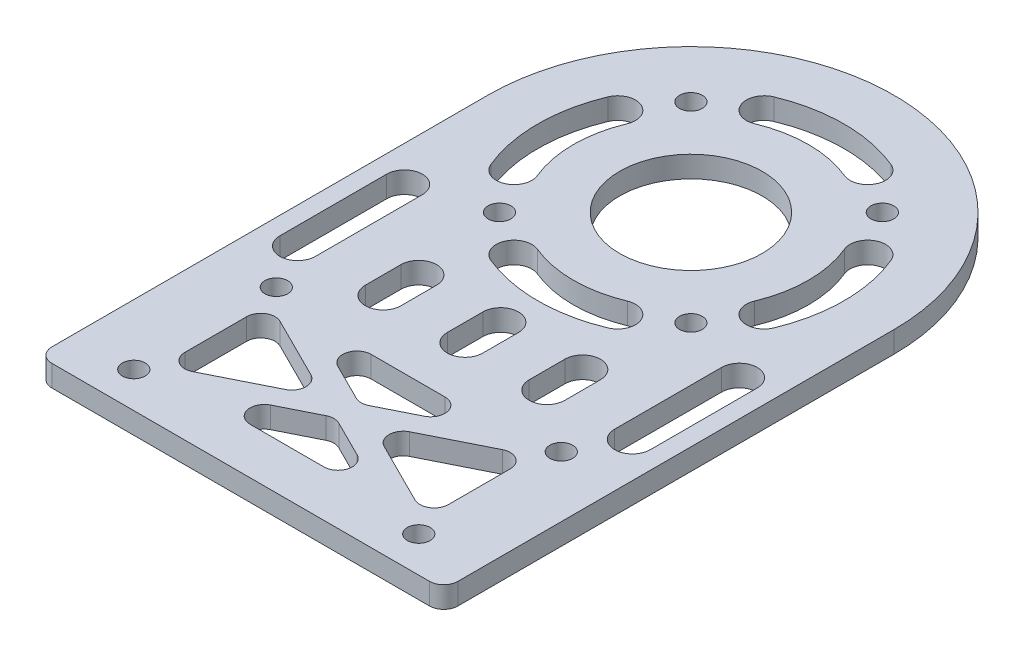
SolidWorks part; units mm, degrees
material "哈碳纤"
ref_plane "前视基准面" through (0, 0, 0) normal (0, 0, 1) x (1, 0, 0)
ref_plane "上视基准面" through (0, 0, 0) normal (0, 1, 0) x (1, 0, 0)
ref_plane "右视基准面" through (0, 0, 0) normal (1, 0, 0) x (0, 0, -1)
other "Configuration Table"
sketch "草图1" plane through (0, 0, 0) normal (0, 1, 0) x (1, 0, 0)
  line L0 (-20, -38.2) -> (20, -58.2) construction
  line L2 (-28.5, 0) -> (-28.5, -63.2)
  line L3 (-28.5, -63.2) -> (28.5, -63.2)
  line L4 (28.5, 0) -> (28.5, -63.2)
  line L5 (-20, -58.2) -> (20, -58.2) construction
  line L6 (-20, -58.2) -> (-20, -38.2) construction
  line L7 (-20, -38.2) -> (20, -38.2) construction
  line L8 (20, -58.2) -> (20, -38.2) construction
  line L9 (-19, 0) -> (0, 0) construction
  line L10 (0, 0) -> (-13.435, 13.435) construction
  arc A0 (28.5, 0) -> (-28.5, 0) centre (0, 0) ccw
  circle A1 centre (-20, -38.2) radius 1.6
  circle A2 centre (20, -38.2) radius 1.6
  circle A3 centre (20, -58.2) radius 1.6
  circle A4 centre (-20, -58.2) radius 1.6
  circle A5 centre (0, 0) radius 19 construction
  circle A6 centre (0, 0) radius 10
  circle A7 centre (-13.435, 13.435) radius 1.6
  circle A8 centre (13.435, 13.435) radius 1.6
  circle A9 centre (13.435, -13.435) radius 1.6
  circle A10 centre (-13.435, -13.435) radius 1.6
  point P10 (0, -48.2)
  dimension "D1" = 57
  dimension "D6" = 3.2
  dimension "D7" = 38
  dimension "D8" = 20
  dimension "D9" = 3.2
  dimension "D2" = 48.2
  dimension "D3" = 15
  dimension "D4" = 40
  dimension "D5" = 20
  dimension "D11" = 45
  dimension "D10" = 4
extrude "凸台-拉伸1" add sketch "草图1" along normal blind 3
sketch "草图2" plane through (0, 3, 0) normal (0, 1, 0) x (1, 0, 0)
  line L0 (-20, -59.7) -> (20, -59.7)
  line L1 (-20, -58.2) -> (20, -58.2)
  line L2 (-20, -58.2) -> (-20, -38.2)
  line L3 (-20, -38.2) -> (20, -38.2)
  line L4 (20, -58.2) -> (20, -38.2)
  line L5 (-20, -58.2) -> (20, -38.2)
  line L6 (-20, -38.2) -> (20, -58.2)
  line L7 (-18.5, -58.2) -> (-18.5, -38.2)
  line L8 (-20, -39.7) -> (20, -39.7)
  line L9 (21.5, -58.2) -> (21.5, -38.2)
  line L10 (-19.3292, -59.5416) -> (20.6708, -39.5416)
  line L11 (-20.6708, -39.5416) -> (19.3292, -59.5416)
  line L12 (-20, -56.7) -> (20, -56.7)
  line L13 (-21.5, -58.2) -> (-21.5, -38.2)
  line L14 (-20, -36.7) -> (20, -36.7)
  line L15 (18.5, -58.2) -> (18.5, -38.2)
  line L16 (-20.6708, -56.8584) -> (19.3292, -36.8584)
  line L17 (-19.3292, -36.8584) -> (20.6708, -56.8584)
  line L18 (-7.271, 17.5537) -> (0, 0) construction
  line L19 (0, 0) -> (7.271, 17.5537) construction
  line L20 (-23.5, -16.7) -> (-23.5, -31.7) construction
  line L21 (-21, -16.7) -> (-21, -31.7)
  line L22 (-26, -16.7) -> (-26, -31.7)
  line L23 (-11.5, -26.7) -> (-11.5, -31.7) construction
  line L24 (-9, -26.7) -> (-9, -31.7)
  line L25 (-14, -26.7) -> (-14, -31.7)
  line L26 (-28.5, 0) -> (-28.5, -63.2) construction
  line L27 (0, 0) -> (0, -48.2) construction
  line L28 (23.5, -16.7) -> (23.5, -31.7) construction
  line L29 (21, -16.7) -> (21, -31.7)
  line L30 (26, -16.7) -> (26, -31.7)
  line L31 (11.5, -26.7) -> (11.5, -31.7) construction
  line L32 (9, -26.7) -> (9, -31.7)
  line L33 (14, -26.7) -> (14, -31.7)
  line L34 (0, -26.7) -> (0, -31.7) construction
  line L35 (2.5, -26.7) -> (2.5, -31.7)
  line L36 (-2.5, -26.7) -> (-2.5, -31.7)
  arc A0 (-20, -59.7) -> (-20, -56.7) centre (-20, -58.2) cw
  arc A1 (20, -59.7) -> (20, -56.7) centre (20, -58.2) ccw
  arc A2 (-18.5, -58.2) -> (-21.5, -58.2) centre (-20, -58.2) cw
  arc A3 (-18.5, -38.2) -> (-21.5, -38.2) centre (-20, -38.2) ccw
  arc A4 (-20, -39.7) -> (-20, -36.7) centre (-20, -38.2) cw
  arc A5 (20, -39.7) -> (20, -36.7) centre (20, -38.2) ccw
  arc A6 (21.5, -58.2) -> (18.5, -58.2) centre (20, -58.2) cw
  arc A7 (21.5, -38.2) -> (18.5, -38.2) centre (20, -38.2) ccw
  arc A8 (-19.3292, -59.5416) -> (-20.6708, -56.8584) centre (-20, -58.2) cw
  arc A9 (20.6708, -39.5416) -> (19.3292, -36.8584) centre (20, -38.2) ccw
  arc A10 (-20.6708, -39.5416) -> (-19.3292, -36.8584) centre (-20, -38.2) cw
  arc A11 (19.3292, -59.5416) -> (20.6708, -56.8584) centre (20, -58.2) ccw
  circle A12 centre (0, 0) radius 19 construction
  arc A13 (-7.271, 17.5537) -> (7.271, 17.5537) centre (0, 0) cw construction
  arc A14 (8.2277, 19.8634) -> (-8.2277, 19.8634) centre (0, 0) ccw
  arc A15 (6.3143, 15.244) -> (-6.3143, 15.244) centre (0, 0) ccw
  arc A16 (6.3143, 15.244) -> (8.2277, 19.8634) centre (7.271, 17.5537) ccw
  arc A17 (-8.2277, 19.8634) -> (-6.3143, 15.244) centre (-7.271, 17.5537) ccw
  arc A18 (17.5537, 7.271) -> (17.5537, -7.271) centre (0, 0) cw construction
  arc A19 (19.8634, -8.2277) -> (19.8634, 8.2277) centre (0, 0) ccw
  arc A20 (15.244, -6.3143) -> (15.244, 6.3143) centre (0, 0) ccw
  arc A21 (15.244, -6.3143) -> (19.8634, -8.2277) centre (17.5537, -7.271) ccw
  arc A22 (19.8634, 8.2277) -> (15.244, 6.3143) centre (17.5537, 7.271) ccw
  arc A23 (7.271, -17.5537) -> (-7.271, -17.5537) centre (0, 0) cw construction
  arc A24 (-8.2277, -19.8634) -> (8.2277, -19.8634) centre (0, 0) ccw
  arc A25 (-6.3143, -15.244) -> (6.3143, -15.244) centre (0, 0) ccw
  arc A26 (-6.3143, -15.244) -> (-8.2277, -19.8634) centre (-7.271, -17.5537) ccw
  arc A27 (8.2277, -19.8634) -> (6.3143, -15.244) centre (7.271, -17.5537) ccw
  arc A28 (-17.5537, -7.271) -> (-17.5537, 7.271) centre (0, 0) cw construction
  arc A29 (-19.8634, 8.2277) -> (-19.8634, -8.2277) centre (0, 0) ccw
  arc A30 (-15.244, 6.3143) -> (-15.244, -6.3143) centre (0, 0) ccw
  arc A31 (-15.244, 6.3143) -> (-19.8634, 8.2277) centre (-17.5537, 7.271) ccw
  arc A32 (-19.8634, -8.2277) -> (-15.244, -6.3143) centre (-17.5537, -7.271) ccw
  arc A33 (-21, -16.7) -> (-26, -16.7) centre (-23.5, -16.7) ccw
  arc A34 (-26, -31.7) -> (-21, -31.7) centre (-23.5, -31.7) ccw
  arc A35 (-9, -26.7) -> (-14, -26.7) centre (-11.5, -26.7) ccw
  arc A36 (-14, -31.7) -> (-9, -31.7) centre (-11.5, -31.7) ccw
  arc A37 (21, -16.7) -> (26, -16.7) centre (23.5, -16.7) cw
  arc A38 (26, -31.7) -> (21, -31.7) centre (23.5, -31.7) cw
  arc A39 (9, -26.7) -> (14, -26.7) centre (11.5, -26.7) cw
  arc A40 (14, -31.7) -> (9, -31.7) centre (11.5, -31.7) cw
  arc A41 (2.5, -26.7) -> (-2.5, -26.7) centre (0, -26.7) ccw
  arc A42 (-2.5, -31.7) -> (2.5, -31.7) centre (0, -31.7) ccw
  point P0 (0, -48.2)
  point P37 (0, 19)
  point P48 (19, 0)
  point P55 (0, -19)
  point P62 (-19, 0)
  point P67 (-23.5, -24.2)
  point P72 (-11.5, -29.2)
  point P84 (23.5, -24.2)
  point P91 (11.5, -29.2)
  point P98 (0, -29.2)
  point P103 (0, 0)
  point P104 (0, -27.5803)
  point P105 (0, -24.1)
  point P106 (-11.5, -24.1)
  point P107 (0, 0)
  point P108 (0, -24.1)
  point P109 (11.5, -24.1)
  point P110 (0, 0)
  point P111 (0, 0)
  point P112 (0, -26.0054)
  point P113 (-23.5, -23.2337)
  point P114 (0, 0)
  dimension "D3" = 38
  dimension "D4" = 45
  dimension "D5" = 5
  dimension "D1" = 1.5
  dimension "D2" = 1.5
  dimension "D7" = 12
  dimension "D8" = 5
  dimension "D9" = 5
  dimension "D10" = 15
  dimension "D11" = 5
  dimension "D12" = 19
  dimension "D6" = 4
extrude "切除-拉伸1" cut sketch "草图2" against normal blind 3 contours L7 L16 L11 | L8 L17 L16 | L10 L17 L15 | L10 L12 L11 | L36 A42 L35 A41 | A40 L33 A39 L32 | A38 L30 A37 L29 | A24 A27 A25 A26 | L25 A36 L24 A35 | L22 A34 L21 A33 | A29 A32 A30 A31 | A19 A22 A20 A21 | A14 A17 A15 A16
fillet "圆角1" radius 2 14 edges at (18.5, 1.5, 40.6271) (18.5, 1.5, 55.7729) (3.3541, 1.5, 48.2) (0, 1.5, 49.8771) (13.6459, 1.5, 56.7) (-13.6459, 1.5, 56.7) (-18.5, 1.5, 40.6271) (-3.3541, 1.5, 48.2) (-18.5, 1.5, 55.7729) (0, 1.5, 46.5229) (-13.6459, 1.5, 39.7) (13.6459, 1.5, 39.7) (-28.5, 1.5, 63.2) (28.5, 1.5, 63.2)
